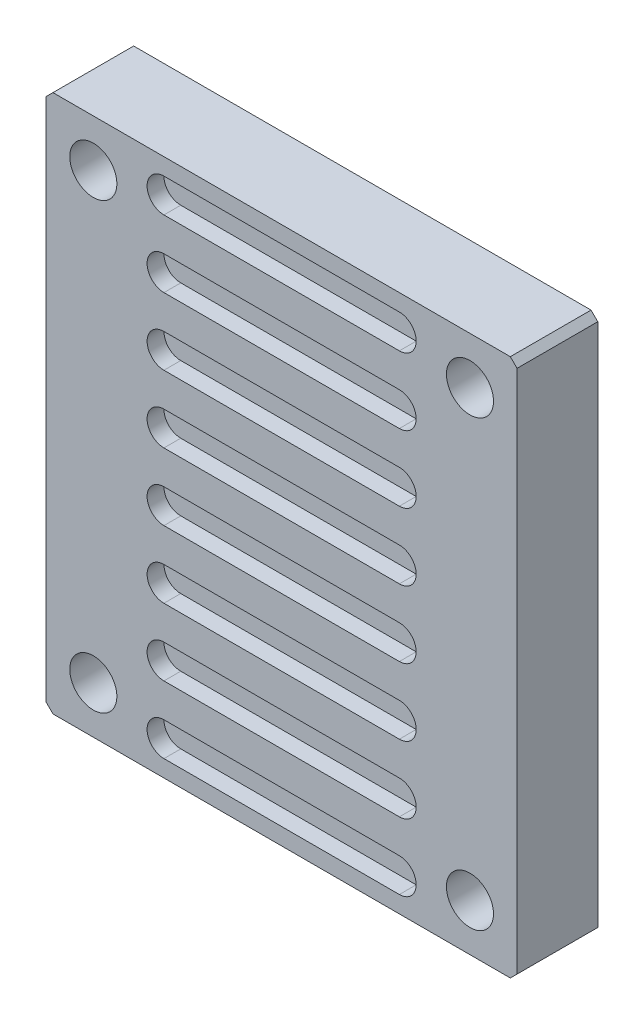
from build123d import *

# Parameters (mm, degrees)
SKETCH_1_W             = 70
SKETCH_1_H             = 80
EXTRUDE_1_DEPTH        = 12
CHAMFER_1_SIZE         = 1
CUT_EXTRUDE_1_DEPTH    = 2.5
PATTERN_LINEAR_1_COUNT = 8
PATTERN_LINEAR_1_PITCH = 10
HOLE_WIZARD_7_0_7_1_D  = 7


with BuildPart() as part:
    # 草图1 → 凸台-拉伸1 (new body)
    with BuildSketch(Plane.XY):
        with Locations((35, -40)):
            Rectangle(SKETCH_1_W, SKETCH_1_H)
    extrude(amount=EXTRUDE_1_DEPTH)

    # 倒角1
    chamfer_1_edges = [part.edges().sort_by_distance(p)[0] for p in [
        (0, 0, 6),
        (70, 0, 6),
        (70, -80, 6),
        (0, -80, 6),
    ]]
    chamfer(chamfer_1_edges, length=CHAMFER_1_SIZE)

    # 草图2 → 切除-拉伸1 (cut)
    with BuildSketch(Plane.XY.offset(12)):
        with BuildLine():
            Line((17.5, -2.5), (52.5, -2.5))
            ThreePointArc((52.5, -2.5), (55, -5), (52.5, -7.5))
            Line((52.5, -7.5), (17.5, -7.5))
            ThreePointArc((17.5, -7.5), (15, -5), (17.5, -2.5))
        make_face()
    cut_extrude_1 = extrude(amount=-CUT_EXTRUDE_1_DEPTH, mode=Mode.SUBTRACT)

    # 阵列(线性)1: 切除-拉伸1 ×8
    with Locations(*[(0, -i * PATTERN_LINEAR_1_PITCH, 0) for i in range(1, PATTERN_LINEAR_1_COUNT)]):
        add(cut_extrude_1, mode=Mode.SUBTRACT)

    # Ø7.0 (7) 直径孔1 (through all)
    with Locations(Plane(origin=(0, 0, 0), x_dir=(-1, 0, 0), z_dir=(0, 0, -1))):
        with Locations((-7, -73), (-7, -7), (-63, -73), (-63, -7)):
            Hole(HOLE_WIZARD_7_0_7_1_D / 2)


solid = part.part
